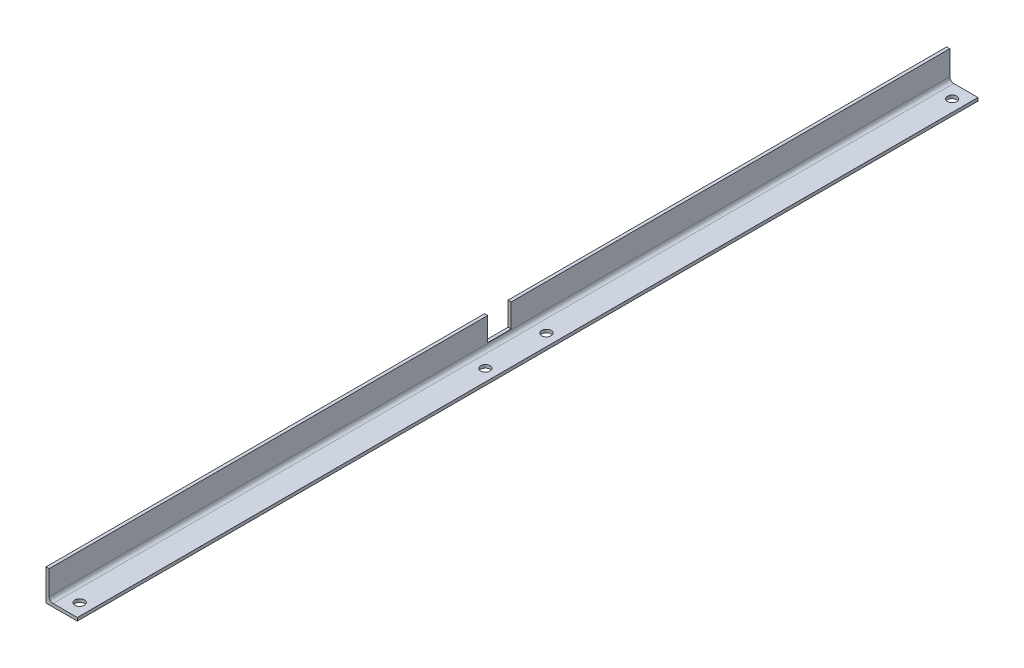
SolidWorks part; units mm, degrees
material "Q235"
ref_plane "前视基准面" through (0, 0, 0) normal (0, 0, 1) x (1, 0, 0)
ref_plane "上视基准面" through (0, 0, 0) normal (0, 1, 0) x (1, 0, 0)
ref_plane "右视基准面" through (0, 0, 0) normal (1, 0, 0) x (0, 0, -1)
sketch "草图1" plane through (0, 0, 0) normal (0, 0, 1) x (1, 0, 0)
  line L0 (0, 0) -> (0, 40)
  line L1 (0, 40) -> (3.99, 40)
  line L2 (4, 39.99) -> (4, 9)
  line L3 (9, 4) -> (39.99, 4)
  line L4 (40, 3.99) -> (40, 0)
  line L5 (40, 0) -> (0, 0)
  arc A0 (4, 39.99) -> (3.99, 40) centre (3.99, 39.99) ccw
  arc A1 (9, 4) -> (4, 9) centre (9, 9) cw
  arc A2 (40, 3.99) -> (39.99, 4) centre (39.99, 3.99) ccw
  point P9 (4, 40)
  point P14 (40, 4)
extrude "拉伸1" add sketch "草图1" along normal blind 1150
hole_wizard "Ø12.0 (12) 直径孔1" positions "草图3" profile "草图2" hole size "Ø12.0" standard "Gb" end condition through all
sketch "草图3" plane through (0, 4, 0) normal (0, 1, 0) x (1, 0, 0)
  line L0 (39.99, -1150) -> (39.99, 0) construction
  line L2 (39.99, -1150) -> (9, -1150) construction
  point P0 (24.99, -1132)
  point P2 (24.99, -614)
  point P4 (24.99, -536)
  point P6 (24.99, -18)
  dimension "D1" = 15
  dimension "D2" = 18
  dimension "D3" = 518
  dimension "D4" = 15
  dimension "D5" = 78
  dimension "D6" = 518
  dimension "D7" = 15
sketch "草图2" plane through (24.99, 4, 1132) normal (1, 0, 0) x (0, 0, 1)
  line L0 (0, 0) -> (0, 4)
  line L1 (0, 4) -> (6, 4)
  line L2 (6, 4) -> (6, 0)
  line L5 (6, 0) -> (0, 0)
  line L11 (0, -6.35) -> (0, 107.95) construction
  dimension "通孔孔直径" = 12
  dimension "通孔孔深度" = 4
ref_plane "基准面1" through (0, 0, 575) normal (0, 0, 1) x (1, 0, 0)
sketch "草图4" plane through (4, 0, 0) normal (1, 0, 0) x (0, 0, -1)
  line L0 (-575, 22) -> (-575, -22) construction
  line L1 (-590, 60.4807) -> (-560, 60.4807)
  line L2 (-590, 60.4807) -> (-590, 10)
  line L3 (-590, 10) -> (-560, 10)
  line L4 (-560, 60.4807) -> (-560, 10)
  line L5 (-1150, 40) -> (0, 40) construction
  dimension "D1" = 30
  dimension "D2" = 15
  dimension "D3" = 30
extrude "切除-拉伸1" cut sketch "草图4" against normal blind 10
equation "\"D2@草图1\" = \"D1@草图1\""
equation "\"D4@草图1\" = \"D3@草图1\""
equation "\"D7@草图1\" = \"D5@草图1\""
